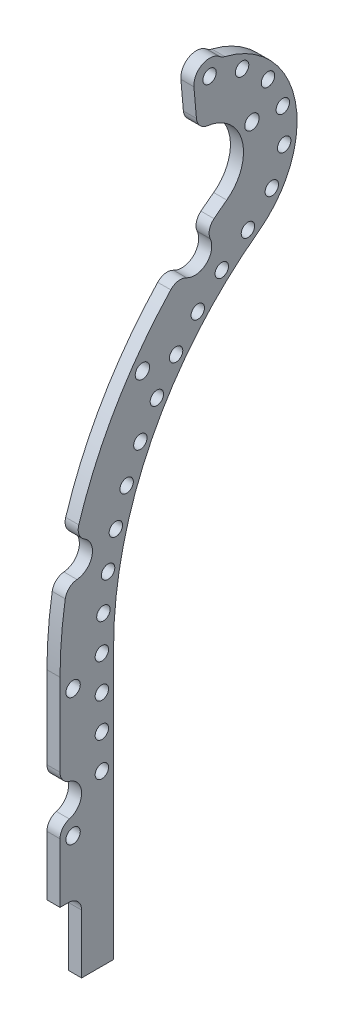
SolidWorks part; units mm, degrees
material "Thornel Mat VMA"
ref_plane "前视基准面" through (0, 0, 0) normal (0, 0, 1) x (1, 0, 0)
ref_plane "上视基准面" through (0, 0, 0) normal (0, 1, 0) x (1, 0, 0)
ref_plane "右视基准面" through (0, 0, 0) normal (1, 0, 0) x (0, 0, -1)
sketch "弹链路径" plane through (0, 0, 0) normal (1, 0, 0) x (0, 0, -1)
  line L0 (0, -41.5) -> (0, 0)
  line L1 (0, 80) -> (6.1652, 79.4606)
  line L2 (0, 80) -> (3.3166, 80) construction
  line L3 (7.1501, 90.7176) -> (5.1803, 68.2036) construction
  arc A0 (18.3088, 36.2295) -> (0, 0) centre (45, 0) ccw
  arc A1 (18.3088, 36.2295) -> (6.1652, 79.4606) centre (4.0735, 55.5519) ccw
  point P11 (6.1652, 79.4606)
  dimension "D1" = 45
  dimension "D2" = 24
  dimension "D3" = 5
  dimension "D4" = 80
  dimension "D5" = 121.5
  dimension "D6" = 22.6
sketch "螺纹孔位" plane through (0, 0, 0) normal (1, 0, 0) x (0, 0, -1)
  line L0 (4.0735, 55.5519) -> (39.5805, 76.0519) construction
  line L1 (4.0735, 55.5519) -> (45.0735, 55.5519) construction
  line L2 (4.0735, 55.5519) -> (39.5805, 35.0519) construction
  line L3 (45, 0) -> (0, 0) construction
  line L4 (-17, -17) -> (17, -17) construction
  line L5 (0, -41.5) -> (0, 0) construction
  line L6 (-15.3402, 14.25) -> (17.1065, 2.4404) construction
  line L7 (2.9189, 45.5322) -> (27.0019, 21.4492) construction
  line L8 (45, 0) -> (27.0019, 21.4492) construction
  line L9 (45, 0) -> (17.1065, 2.4404) construction
  arc A0 (39.5805, 76.0519) -> (39.5805, 35.0519) centre (4.0735, 55.5519) cw construction
  circle A1 centre (39.5805, 76.0519) radius 1.5
  circle A2 centre (39.5805, 35.0519) radius 1.5
  circle A3 centre (45.0735, 55.5519) radius 1.5
  circle A4 centre (-17, -17) radius 1.5
  circle A5 centre (17, -17) radius 1.5
  arc A6 (-15.3402, 14.25) -> (2.9189, 45.5322) centre (45, 0) cw construction
  arc A7 (17.1065, 2.4404) -> (27.0019, 21.4492) centre (45, 0) cw construction
  circle A8 centre (-15.3402, 14.25) radius 1.5
  circle A9 centre (2.9189, 45.5322) radius 1.5
  circle A10 centre (27.0019, 21.4492) radius 1.5
  circle A11 centre (17.1065, 2.4404) radius 1.5
  point P10 (0, -17)
  dimension "D1" = 41
  dimension "D3" = 62
  dimension "D4" = 28
  dimension "D11" = 3
  dimension "D2" = 30
  dimension "D5" = 175
  dimension "D6" = 165
  dimension "D7" = 5
  dimension "D8" = 45
  dimension "D9" = 17
  dimension "D10" = 34
sketch "草图3" plane through (0, 0, 0) normal (1, 0, 0) x (0, 0, -1)
  line L0 (-19.5, 0) -> (-19.5, -25) construction
  line L1 (-19.5, -25) -> (-14.1, -25) construction
  line L2 (-14.1, -25) -> (-14.1, 0) construction
  line L3 (7.2554, 58.7339) -> (11.0738, 62.5523) construction
  line L4 (4.0735, 55.5519) -> (45.0735, 55.5519) construction
  line L5 (4.0735, 55.5519) -> (13.9735, 55.5519) construction
  line L6 (-17.7, 0) -> (-17.7, -14.496)
  line L10 (-17.7, -19.504) -> (-17.7, -30.5)
  line L13 (-17.7, 0) -> (-17.7, -30.5) construction
  line L14 (-17.7, -30.5) -> (-14.4, -30.5)
  line L15 (-14.4, -30.5) -> (-14.4, -41.5)
  line L16 (-15.7, 0) -> (-15.7, -30.5) construction
  line L17 (-14.4, -41.5) -> (-9.5, -41.5)
  line L18 (-9.5, -41.5) -> (-9.5, 0)
  line L19 (-11.3, -10.4226) -> (-11.3, -15.6226) construction
  line L20 (5.1803, 68.2036) -> (10.158, 66.6995) construction
  line L21 (10.158, 66.6995) -> (14.1157, 63.3265) construction
  line L22 (14.1157, 63.3265) -> (16.3898, 58.6501) construction
  line L23 (16.3898, 58.6501) -> (16.599, 53.4543) construction
  line L24 (16.599, 53.4543) -> (14.7084, 48.6102) construction
  line L25 (14.7084, 48.6102) -> (11.0516, 44.9132) construction
  line L26 (11.0516, 44.9132) -> (7.0525, 41.5894) construction
  line L27 (7.0525, 41.5894) -> (3.3772, 37.9109) construction
  line L28 (3.3772, 37.9109) -> (0.0569, 33.9089) construction
  line L29 (0.0569, 33.9089) -> (-2.8799, 29.6176) construction
  line L30 (-2.8799, 29.6176) -> (-5.4083, 25.0737) construction
  line L31 (-5.4083, 25.0737) -> (-7.5067, 20.3159) construction
  line L32 (-7.5067, 20.3159) -> (-9.1572, 15.3848) construction
  line L33 (-9.1572, 15.3848) -> (-10.3456, 10.3224) construction
  line L34 (-10.3456, 10.3224) -> (-11.0619, 5.172) construction
  line L35 (-11.0619, 5.172) -> (-11.3, -0.0226) construction
  line L36 (-11.3, -0.0226) -> (-11.3, -5.2226) construction
  line L37 (-11.3, -5.2226) -> (-11.3, -10.4226) construction
  line L38 (-11.3, 0) -> (-11.3, -41.5) construction
  line L39 (3.3307, 61.808) -> (2.7895, 67.9944)
  arc A1 (0.6293, 44.3004) -> (4.3271, 47.7179) centre (2.9189, 45.5322) ccw
  arc A2 (-16.5509, 11.9491) -> (-15.3936, 16.8495) centre (-15.3402, 14.25) ccw
  arc A3 (-17.7, -19.504) -> (-17.7, -14.496) centre (-17, -17) ccw
  arc A4 (0.6293, 44.3004) -> (-15.3936, 16.8495) centre (45, 0) ccw
  circle A5 centre (2.9189, 45.5322) radius 1.5 construction
  circle A6 centre (-15.3402, 14.25) radius 1.5 construction
  arc A7 (7.8102, 50.4798) -> (-17.7, 0) centre (45, 0) ccw construction
  arc A8 (-16.5509, 11.9491) -> (-17.7, 0) centre (45, 0) ccw
  circle A9 centre (-17, -17) radius 1.5 construction
  circle A14 centre (2.9189, 45.5322) radius 1.5 construction
  circle A15 centre (-15.3402, 14.25) radius 1.5 construction
  circle A18 centre (-17, -17) radius 1.5 construction
  arc A19 (9.9455, 47.5814) -> (-14.1, 0) centre (45, 0) ccw construction
  arc A20 (6.7426, 51.929) -> (-19.5, 0) centre (45, 0) ccw construction
  arc A21 (6.7426, 51.929) -> (7.2554, 58.7339) centre (4.0735, 55.5519) ccw construction
  arc A22 (9.9455, 47.5814) -> (11.0738, 62.5523) centre (4.0735, 55.5519) ccw construction
  arc A23 (7.8102, 50.4798) -> (4.3271, 47.7179) centre (45, 0) ccw
  arc A24 (7.8102, 50.4798) -> (3.3307, 61.808) centre (4.0735, 55.5519) ccw
  arc A34 (12.674, 43.878) -> (-9.5, 0) centre (45, 0) ccw
  arc A36 (8.9965, 48.8696) -> (9.9424, 61.4209) centre (4.0735, 55.5519) ccw construction
  arc A37 (8.9965, 48.8696) -> (-15.7, 0) centre (45, 0) ccw construction
  arc A38 (12.674, 43.878) -> (7.0154, 69.7503) centre (4.0735, 55.5519) ccw
  circle A39 centre (5.1803, 68.2036) radius 1.025
  circle A40 centre (-15.7, -22) radius 1.1
  circle A41 centre (-15.7, -2.5) radius 1.1
  circle A42 centre (-5.0929, 34.2811) radius 1.1
  circle A43 centre (11.667, 58.9028) radius 1.1
  arc A44 (11.6063, 45.3272) -> (-11.3, 0) centre (45, 0) ccw construction
  arc A45 (11.6063, 45.3272) -> (4.1565, 68.2517) centre (4.0735, 55.5519) ccw construction
  circle A46 centre (-15.7, -22) radius 2.35 construction
  circle A47 centre (10.158, 66.6995) radius 1.025
  circle A48 centre (14.1157, 63.3265) radius 1.025
  circle A49 centre (16.3898, 58.6501) radius 1.025
  circle A50 centre (16.599, 53.4543) radius 1.025
  circle A51 centre (14.7084, 48.6102) radius 1.025
  circle A52 centre (11.0516, 44.9132) radius 1.025
  circle A53 centre (7.0525, 41.5894) radius 1.025
  circle A54 centre (3.3772, 37.9109) radius 1.025
  circle A55 centre (0.0569, 33.9089) radius 1.025
  circle A56 centre (-2.8799, 29.6176) radius 1.025
  circle A57 centre (-5.4083, 25.0737) radius 1.025
  circle A58 centre (-7.5067, 20.3159) radius 1.025
  circle A59 centre (-9.1572, 15.3848) radius 1.025
  circle A60 centre (-10.3456, 10.3224) radius 1.025
  circle A61 centre (-11.0619, 5.172) radius 1.025
  circle A62 centre (-11.3, -0.0226) radius 1.025
  circle A63 centre (-11.3, -5.2226) radius 1.025
  circle A64 centre (-11.3, -10.4226) radius 1.025
  circle A66 centre (-11.3, -15.6226) radius 1.025
  circle A67 centre (-11.3, -0.0226) radius 1.85 construction
  circle A68 centre (-11.3, -5.2226) radius 1.85 construction
  circle A69 centre (-15.7, -2.5) radius 2.35 construction
  arc A70 (7.8102, 50.4798) -> (8.5282, 60.0067) centre (4.0735, 55.5519) ccw construction
  arc A71 (8.9965, 48.8696) -> (9.9424, 61.4209) centre (4.0735, 55.5519) ccw construction
  arc A72 (7.0154, 69.7503) -> (2.7895, 67.9944) centre (5.1803, 68.2036) ccw
  point P45 (0, 0)
  point P46 (0, 80)
  point P87 (0, 0)
  point P98 (0, 0)
  dimension "D1" = 64.5
  dimension "D3" = 59.1
  dimension "D5" = 1.8
  dimension "D6" = 5.2
  dimension "D7" = 13.5
  dimension "D10" = 11.3
  dimension "D16" = 2.2
  dimension "D9" = 2.05
  dimension "D11" = 4.7
  dimension "D12" = 5.2
  dimension "D15" = 3.7
  dimension "D22" = 2.4
  dimension "D2" = 8
  dimension "D4" = 45
  dimension "D8" = 11
  dimension "D14" = 1.8
  dimension "D17" = 3
  dimension "D18" = 3
  dimension "D19" = 14.5
  dimension "D20" = 22.5
  dimension "D21" = 5.2
  dimension "D23" = 85
  dimension "D13" = 2
extrude "凸台-拉伸1" add sketch "草图3" along normal mid plane 2 contours L0 L1 L2 A19 A22 L3 A21 A20 | A40
fillet "R2 圆角1" radius 2 9 edges at (0, 69.7503, -7.0154) (0, 61.808, -3.3307) (0, 47.7179, -4.3271) (0, 44.3004, -0.6293) (0, 16.8495, 15.3936) (0, 11.9491, 16.5509) (0, -14.496, 17.7) (0, -19.504, 17.7) (0, -30.5, 14.4)
